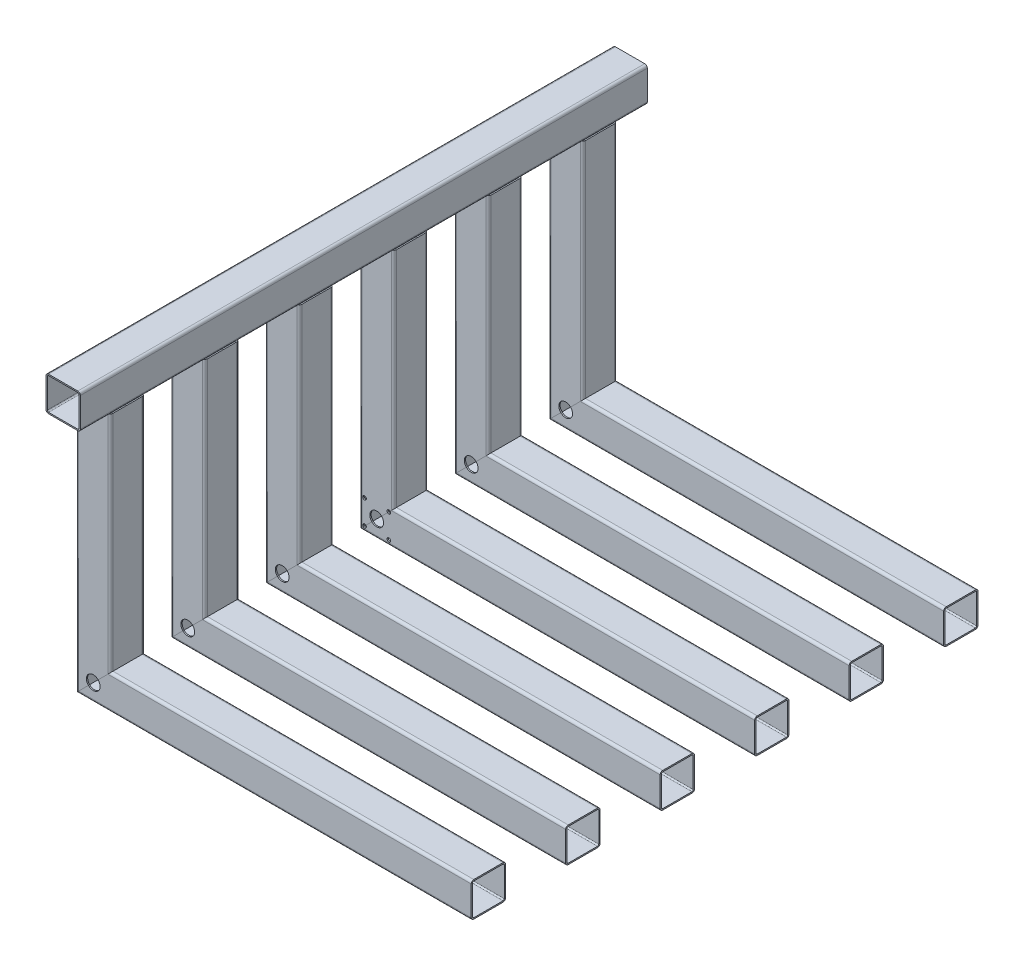
SolidWorks part; units mm, degrees
material "Q235-A"
ref_plane "前视基准面" through (0, 0, 0) normal (0, 0, 1) x (1, 0, 0)
ref_plane "上视基准面" through (0, 0, 0) normal (0, 1, 0) x (1, 0, 0)
ref_plane "右视基准面" through (0, 0, 0) normal (1, 0, 0) x (0, 0, -1)
sketch "草图1" plane through (0, 0, 0) normal (0, 1, 0) x (1, 0, 0)
  line L1 (-220, 330) -> (220, 330)
  line L2 (-220, 330) -> (-220, -330)
  line L3 (-220, -330) -> (220, -330)
  line L4 (220, 330) -> (220, -330)
  line L5 (-220, 330) -> (220, -330) construction
  line L6 (-220, -330) -> (220, 330) construction
  point P0 (0, 0)
  dimension "D1" = 660
  dimension "D2" = 440
sketch3d "3D草图1"
  line L0 (-220, 0, -330) -> (-220, 0, 330) construction
  line L1 (-220, 0, 330) -> (220, 0, 330) construction
  line L2 (220, 0, -330) -> (220, 0, 330) construction
  line L3 (-220, 0, -330) -> (220, 0, -330) construction
  line L4 (-220, 0, -330) -> (-220, 0, 330)
  line L5 (-220, 0, 330) -> (220, 0, 330)
  line L6 (220, 0, -330) -> (220, 0, 330)
  line L7 (-220, 0, -330) -> (220, 0, -330)
  line L8 (-220, 0, 330) -> (-220, 300, 330)
  line L9 (-220, 0, -330) -> (-220, 300, -330)
  line L12 (-220, 300, 330) -> (-220, 300, -330)
  line L13 (-220, 300, 275) -> (-220, 0, 275)
  line L14 (-220, 0, 275) -> (220, 0, 275)
  dimension "D1" = 300
  dimension "D2" = 55
other "冷弯空心方管gb∕t6728-2002 40 X 40 X 1.5(1)"
ref_plane "基准面1" through (-220, 300, 330) normal (0, 0, -1) x (1, 0, 0)
sketch "Sketch1" plane through (-220, 300, 330) normal (0, 0, -1) x (1, 0, 0)
  line L0 (-17, -18.5) -> (17, -18.5)
  line L1 (-18.5, -17) -> (-18.5, 17)
  line L2 (17, 18.5) -> (-17, 18.5)
  line L3 (18.5, 17) -> (18.5, -17)
  line L4 (-17, -20) -> (17, -20)
  line L5 (-20, -17) -> (-20, 17)
  line L6 (17, 20) -> (-17, 20)
  line L7 (20, 17) -> (20, -17)
  arc A0 (20, 17) -> (17, 20) centre (17, 17) ccw
  arc A1 (17, -20) -> (20, -17) centre (17, -17) ccw
  arc A2 (-20, -17) -> (-17, -20) centre (-17, -17) ccw
  arc A3 (-17, 20) -> (-20, 17) centre (-17, 17) ccw
  arc A4 (-17, 18.5) -> (-18.5, 17) centre (-17, 17) ccw
  arc A5 (18.5, 17) -> (17, 18.5) centre (17, 17) ccw
  arc A6 (17, -18.5) -> (18.5, -17) centre (17, -17) ccw
  arc A7 (-18.5, -17) -> (-17, -18.5) centre (-17, -17) ccw
  point P0 (-20, 0)
  point P1 (20, 0)
  point P2 (0, 20)
  point P3 (0, -20)
  point P4 (0, 0)
  point P5 (-20, -20)
  point P6 (20, -20)
  point P7 (20, 20)
  point P8 (-20, 20)
  point P33 (0, 0)
  dimension "D1" = 3
  dimension "Thickness" = 1.5
  dimension "V_leg" = 40
pattern_linear "阵列(线性)1" count 6 spacing 110 along (0, 0, -1) of bodies 130 129 106 107 108
sketch "草图2" plane through (0, 0, 295) normal (0, 0, 1) x (1, 0, 0)
  line L0 (-220, 0) -> (220, 0) construction
  line L2 (-240, -20) -> (-240, 280) construction
  circle A0 centre (-220, 0) radius 8
  dimension "D1" = 16
  dimension "D2" = 20
extrude "切除-拉伸1" cut sketch "草图2" against normal through all
sketch "草图3" plane through (0, 0, 35) normal (0, 0, -1) x (-1, 0, 0)
  line L0 (200, 20) -> (240, 20)
  line L1 (-220, 20) -> (200, 20) construction
  line L2 (203, 17) -> (200, 20) construction
  line L3 (240, -20) -> (240, 280) construction
  line L4 (240, 20) -> (240, -60)
  line L5 (200, 20) -> (200, -60)
  arc A0 (200, -60) -> (240, -60) centre (220, -60) ccw
  circle A1 centre (220, -60) radius 6
  dimension "D1" = 60
  dimension "D2" = 12
base flange "基体-法兰1" [suppressed] sketch "草图3" thickness 5 reverse thickness direction yes parameters "D1"=0
mirror "镜向1" [suppressed] about plane through (0, 0, 0) normal (0, 0, 1)
hole_wizard "M5 螺纹孔1" positions "草图4" profile "草图5" tap size "M5" standard "GB" end condition up to next
sketch "草图4" plane through (0, 0, -35) normal (0, 0, 1) x (1, 0, 0)
  line L0 (-240, 0) -> (-220, 0) construction
  line L1 (-220, 0) -> (-234.1421, 14.1421) construction
  circle A0 centre (-220, 0) radius 20 construction
  point P8 (-234.1421, 14.1421)
  dimension "D1" = 40
  dimension "D2" = 45
sketch "草图5" plane through (-234.1421, 14.1421, -35) normal (1, 0, 0) x (0, -1, 0)
  line L0 (0, 0) -> (0, 1.501)
  line L1 (0, 1.501) -> (2.1, 1.501)
  line L2 (2.1, 1.501) -> (2.1, 0)
  line L5 (2.1, 0) -> (0, 0)
  line L11 (0, -6.35) -> (0, 107.95) construction
  dimension "通孔螺纹孔钻头直径" = 4.2
  dimension "通孔螺纹孔钻头深度" = 1.501
cosmetic thread "孔螺蚊线1"
pattern_circular "阵列(圆周)1" count 4 over 360 about axis through (-220, 0, 0) along (0, 0, 1) of "M5 螺纹孔1"
mirror "镜向2" about plane through (0, 0, 0) normal (0, 0, 1) of "阵列(圆周)1", "M5 螺纹孔1"
sketch "折弯-线1" [suppressed] plane through (0, 0, 0) normal (0, 1, 0) x (1, 0, 0)
sketch "边界框1" [suppressed] plane through (0, 0, 0) normal (0, 1, 0) x (1, 0, 0)
sheet metal parameters "钣金53" thickness 5 parameters "D1"=0
flat pattern "平板型式53"
sketch "折弯-线2" plane through (0, 0, 0) normal (0, 1, 0) x (1, 0, 0)
sketch "边界框2" [suppressed] plane through (0, 0, 0) normal (0, 1, 0) x (1, 0, 0)
sheet metal parameters "钣金54" thickness 5 parameters "D1"=0
flat pattern "平板型式54"
sketch "折弯-线3" plane through (0, 0, 0) normal (0, 1, 0) x (1, 0, 0)
sketch "边界框3" [suppressed] plane through (0, 0, 0) normal (0, 1, 0) x (1, 0, 0)
